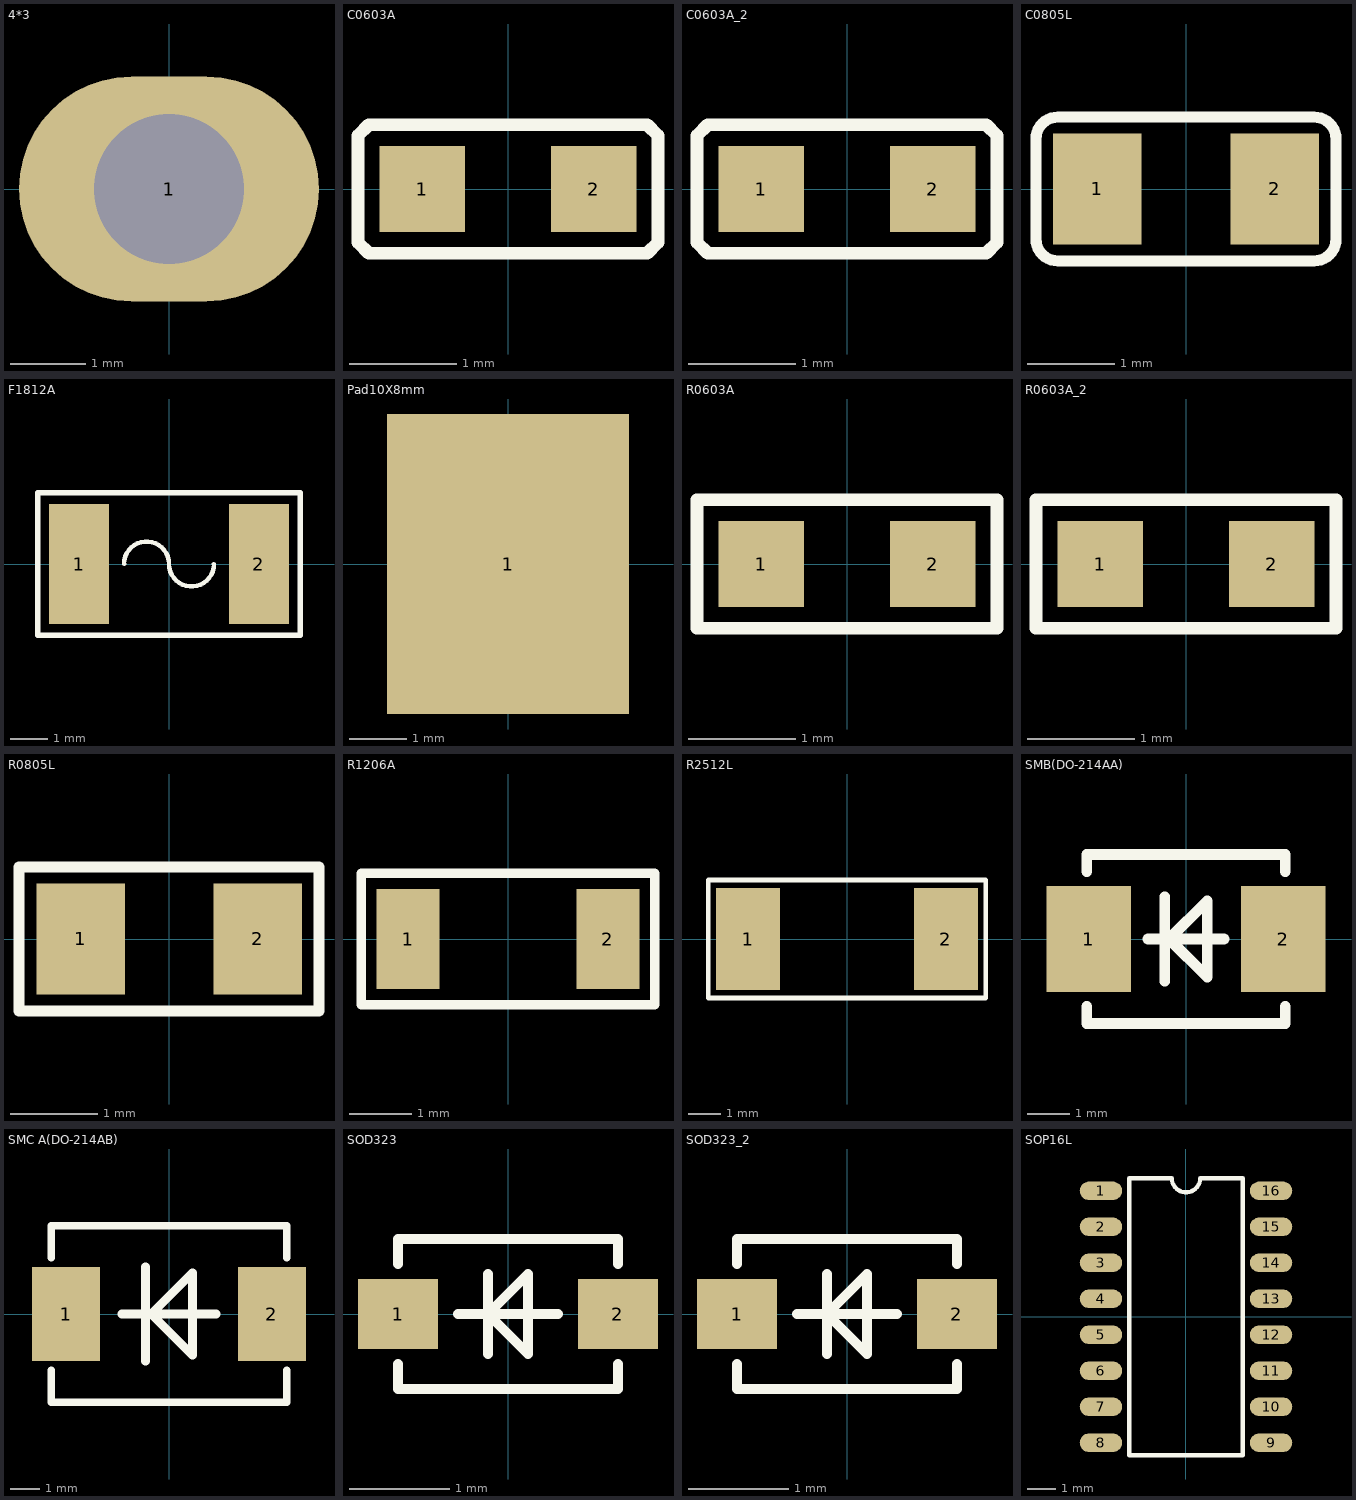
[diagram p0: the footprints below, top view; thin cyan lines are the x and y axes]
# Altium footprint library MISC75736.PcbLib: 19 footprints (part 1 of 2)
Each footprint in its own frame and in the unit in brackets; x right, y up, seen from the top. Pads: shape width x height; smd on the part's side, far side on the other; paste and mask are expansions set on the pad; w line width, h text height; cw(c..) or ccw(c..) is an arc to the next point about the centre after c.

## 4*3 [mm] "through-hole pad"
height 0.5
pads (1):
  oval 4x3 hole 2 mask+0: 1(0,0)

## C0603A [mm] "chip capacitor"
pads (2):
  rect 0.8x0.8 smd mask+0.08: 1(-0.8,0) 2(0.8,0)
Top Overlay:
  lines w0.12: 0.551,-0.6 1.2,-0.6 ; -1.4,-0.5 -1.4,0.5 -1.3,0.6 1.3,0.6 1.4,0.5 1.4,-0.5 1.3,-0.6 -1.3,-0.6 -1.4,-0.5

## C0603A_2 [mm]
pads (2):
  rect 0.8x0.8 smd mask+0.08: 1(-0.8,0) 2(0.8,0)
Top Overlay:
  lines w0.12: 0.551,-0.6 1.2,-0.6 ; -1.4,-0.5 -1.4,0.5 -1.3,0.6 1.3,0.6 1.4,0.5 1.4,-0.5 1.3,-0.6 -1.3,-0.6 -1.4,-0.5

## C0805L [mil] "chip capacitor"
height 19.68
pads (2):
  rect 40x50 smd paste+0 mask+1.97: 1(-40,0) 2(40,0)
Top Overlay:
  lines w5: -67.72,-22.64 ccw(c-57.87,-22.64) -57.87,-32.48 57.87,-32.48 ccw(c57.87,-22.64) 67.72,-22.64 67.72,22.64 ccw(c57.87,22.64) 57.87,32.48 -57.87,32.48 ccw(c-57.87,22.64) -67.72,22.64 -67.72,-22.64

## F1812A [mm] "chip resistor"
height 0.5
pads (2):
  rect 1.6x3.2 smd: 1(-2.4,0) 2(2.4,0)
Top Overlay:
  lines w0.12: -1.2,0 cw(c-0.6,0) 0,0 ccw(c0.6,0) 1.2,0
  lines w0.15: -3.5,-1.9 -3.5,1.9 3.5,1.9 3.5,-1.9 -3.5,-1.9

## Pad10X8mm [mm]
height 0.5
pads (1):
  rect 4.2x5.2 smd: 1(0,0)

## R0603A [mm] "chip resistor"
height 0.5
pads (2):
  rect 0.8x0.8 smd mask+0.08: 1(-0.8,0) 2(0.8,0)
Top Overlay:
  lines w0.12: -1.4,-0.6 1.4,-0.6 1.4,0.6 -1.4,0.6 -1.4,-0.6

## R0603A_2 [mm]
pads (2):
  rect 0.8x0.8 smd mask+0.08: 1(-0.8,0) 2(0.8,0)
Top Overlay:
  lines w0.12: -1.4,-0.6 1.4,-0.6 1.4,0.6 -1.4,0.6 -1.4,-0.6

## R0805L [mil] "chip resistor"
height 19.68
pads (2):
  rect 40x50 smd paste+0 mask+1.97: 1(-40,0) 2(40,0)
Top Overlay:
  lines w5: -67.91,-32.48 -67.91,32.48 ; -67.72,-32.48 67.72,-32.48 67.72,32.48 -67.72,32.48

## R1206A [mm] "chip resistor"
height 0.5
pads (2):
  rect 1x1.6 smd: 1(-1.6,0) 2(1.6,0)
Top Overlay:
  lines w0.15: -2.35,-1.05 -2.35,1.05 2.35,1.05 2.35,-1.05 -2.35,-1.05

## R2512L [mm] "chip resistor"
height 0.5
pads (2):
  rect 2x3.2 smd: 1(-3.1,0) 2(3.1,0)
Top Overlay:
  lines w0.15: -4.35,-1.85 -4.35,1.85 4.35,1.85 4.35,-1.85 -4.35,-1.85

## SMB(DO-214AA) [mm] "chip diode"
height 0.5
pads (2):
  rect 2x2.5 smd: 1(-2.3,0) 2(2.3,0)
Top Overlay:
  lines w0.254: -2.35,-1.6 -2.35,-2 2.35,-2 2.35,-1.6 ; -2.35,1.6 -2.35,2 2.35,2 2.35,1.6 ; -0.9,0 0.9,0 ; -0.5,-1 -0.5,1 ; -0.4,0 0.5,0.9 0.5,-0.9 -0.4,0

## SMC A(DO-214AB) [mm] "chip diode"
pads (2):
  rect 2.3x3.2 smd: 1(-3.5,0) 2(3.5,0)
Top Overlay:
  lines w0.254: -4,-1.905 -4,-3 4,-3 4,-1.905 ; -4,1.905 -4,3 4,3 4,1.905
  lines w0.3: -1.6,0 1.6,0 ; -0.8,-1.6 -0.8,1.6 ; -0.6,0 0.8,1.4 0.8,-1.4 -0.6,0

## SOD323 [mm] "chip diode"
pads (2):
  rect 0.8x0.7 smd: 1(-1.1,0) 2(1.1,0)
Top Overlay:
  lines w0.1: -1.1,-0.5 -1.1,-0.75 1.1,-0.75 1.1,-0.5 ; -1.1,0.5 -1.1,0.75 1.1,0.75 1.1,0.5 ; -0.5,0 0.5,0 ; -0.2,-0.4 -0.2,0.4 ; -0.2,0 0.2,0.4 0.2,-0.4 -0.2,0

## SOD323_2 [mm]
pads (2):
  rect 0.8x0.7 smd: 1(-1.1,0) 2(1.1,0)
Top Overlay:
  lines w0.1: -1.1,-0.5 -1.1,-0.75 1.1,-0.75 1.1,-0.5 ; -1.1,0.5 -1.1,0.75 1.1,0.75 1.1,0.5 ; -0.5,0 0.5,0 ; -0.2,-0.4 -0.2,0.4 ; -0.2,0 0.2,-0.4 0.2,0.4 -0.2,0

## SOP16L [mm]
pads (16):
  oval 1.5x0.65 smd: 1(-3,4.445) 2(-3,3.175) 3(-3,1.905) 4(-3,0.635) 5(-3,-0.635) 6(-3,-1.905) 7(-3,-3.175) 8(-3,-4.445) 9(3,-4.445) 10(3,-3.175) 11(3,-1.905) 12(3,-0.635) 13(3,0.635) 14(3,1.905) 15(3,3.175) 16(3,4.445)
Top Overlay:
  lines w0.15: -2,-4.89 2,-4.89 2,4.89 0.5,4.89 cw(c0,4.89) -0.5,4.89 -2,4.89 -2,-4.89